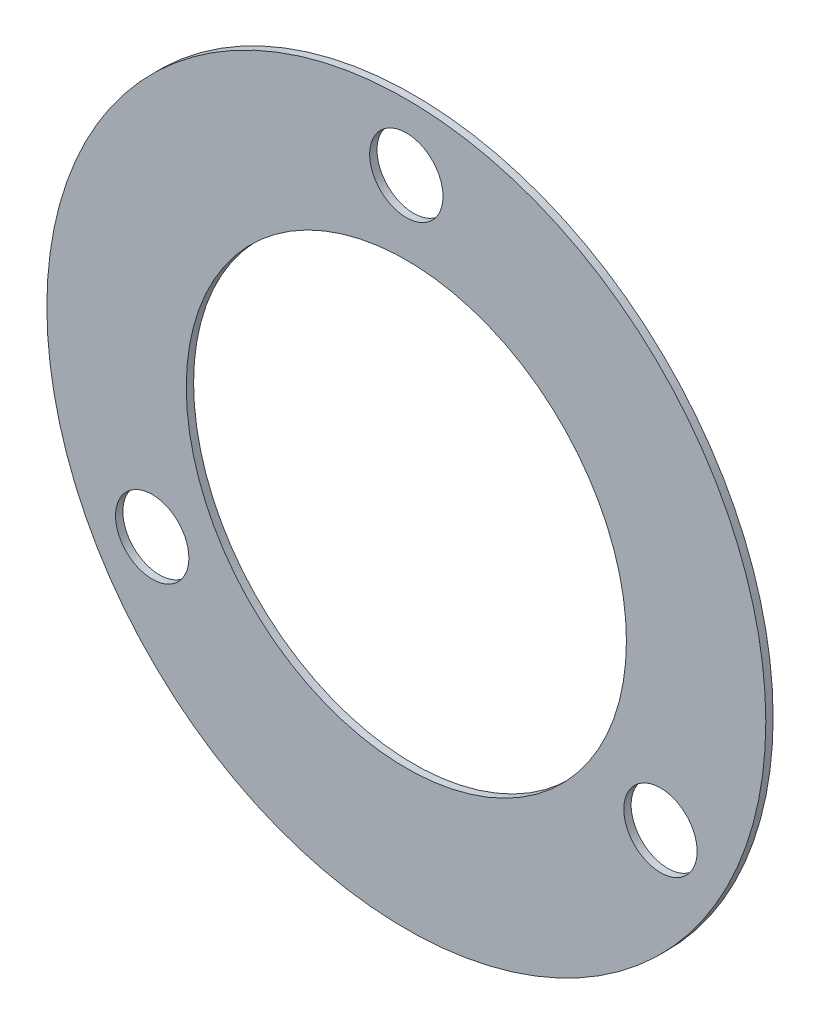
SolidWorks part; units mm, degrees
ref_plane "Front Plane" through (0, 0, 0) normal (0, 0, 1) x (1, 0, 0)
ref_plane "Top Plane" through (0, 0, 0) normal (0, 1, 0) x (1, 0, 0)
ref_plane "Right Plane" through (0, 0, 0) normal (1, 0, 0) x (0, 0, -1)
other "Configuration Table"
sketch "Sketch1" plane through (0, 0, 0) normal (0, 0, 1) x (1, 0, 0)
  circle A0 centre (0, 0) radius 24.5
  circle A1 centre (0, 0) radius 15
  dimension "D1" = 30
  dimension "D2" = 49
extrude "Boss-Extrude1" add sketch "Sketch1" along normal blind 0.5
sketch "Sketch2" plane through (0, 0, 0.5) normal (0, 0, 1) x (1, 0, 0)
  circle A0 centre (0, 0) radius 20 construction
  circle A1 centre (0, 20) radius 2.5
  circle A2 centre (17.3205, -10) radius 2.5
  circle A3 centre (-17.3205, -10) radius 2.5
  point P12 (0, 0)
  dimension "D1" = 40
  dimension "D2" = 5
  dimension "D3" = 3
extrude "Cut-Extrude1" cut sketch "Sketch2" against normal blind 0.5
